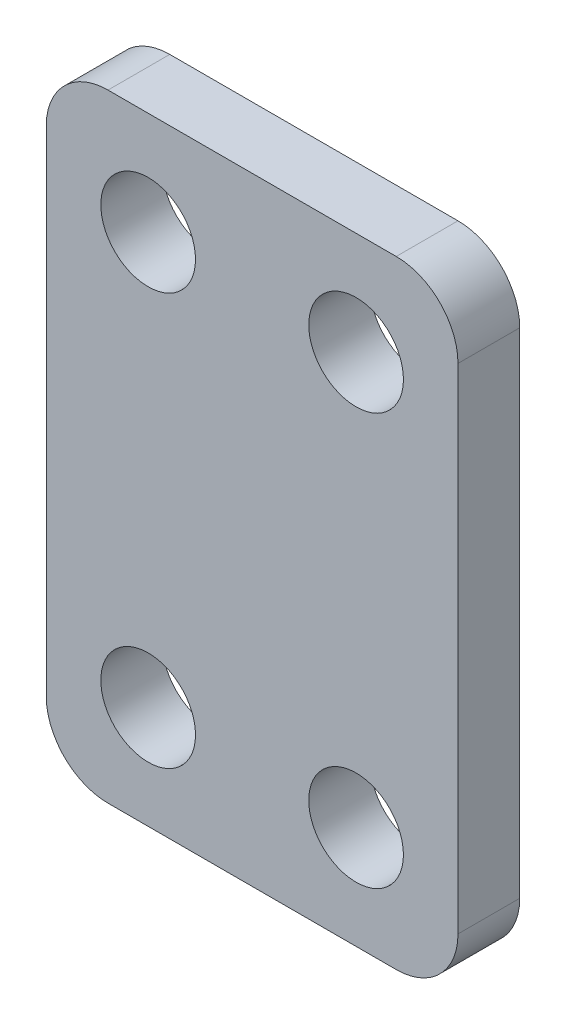
from build123d import *

# Parameters (mm, degrees)
SKETCH1_W           = 20
SKETCH1_H           = 30
BOSS_EXTRUDE1_DEPTH = 3
SKETCH2_R           = 2.3
CUT_EXTRUDE1_DEPTH  = 3
FILLET1_R           = 3


with BuildPart() as part:
    # Sketch1 → Boss-Extrude1 (new body)
    with BuildSketch(Plane.XY):
        Rectangle(SKETCH1_W, SKETCH1_H)
    extrude(amount=BOSS_EXTRUDE1_DEPTH)

    # Sketch2 → Cut-Extrude1 (cut)
    with BuildSketch(Plane.XY.offset(3)):
        with Locations((-5.05, 10)):
            Circle(SKETCH2_R)
        with Locations((5.05, 10)):
            Circle(SKETCH2_R)
        with Locations((-5.05, -10)):
            Circle(SKETCH2_R)
        with Locations((5.05, -10)):
            Circle(SKETCH2_R)
    extrude(amount=-CUT_EXTRUDE1_DEPTH, mode=Mode.SUBTRACT)

    # Fillet1
    fillet1_edges = [part.edges().sort_by_distance(p)[0] for p in [
        (10, -15, 1.5),
        (-10, -15, 1.5),
        (-10, 15, 1.5),
        (10, 15, 1.5),
    ]]
    fillet(fillet1_edges, radius=FILLET1_R)


solid = part.part
